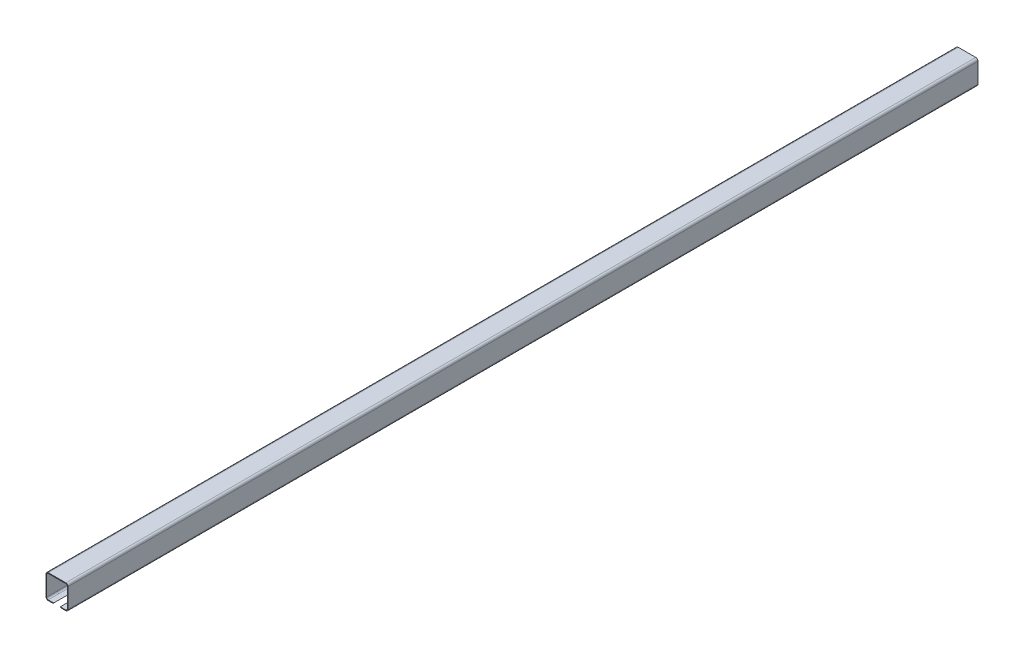
from build123d import *

# Parameters (mm, degrees)
BOSS_EXTRUDE1_DEPTH = 4135


with BuildPart() as part:
    # Sketch1 → Boss-Extrude1 (new body)
    with BuildSketch(Plane.XY):
        with BuildLine():
            Line((-40, 55), (0, 55))
            Line((0, 55), (40, 55))
            ThreePointArc((40, 55), (47.071067812, 52.071067812), (50, 45))
            Line((50, 45), (50, -45))
            ThreePointArc((50, -45), (47.071067812, -52.071067812), (40, -55))
            Line((40, -55), (18, -55))
            Line((18, -55), (15, -52))
            Line((15, -52), (40, -52))
            ThreePointArc((40, -52), (44.949747468, -49.949747468), (47, -45))
            Line((47, -45), (47, 45))
            ThreePointArc((47, 45), (44.949747468, 49.949747468), (40, 52))
            Line((40, 52), (0, 52))
            Line((0, 52), (-40, 52))
            ThreePointArc((-40, 52), (-44.949747468, 49.949747468), (-47, 45))
            Line((-47, 45), (-47, -45))
            ThreePointArc((-47, -45), (-44.949747468, -49.949747468), (-40, -52))
            Line((-40, -52), (-15, -52))
            Line((-15, -52), (-18, -55))
            Line((-18, -55), (-40, -55))
            ThreePointArc((-40, -55), (-47.071067812, -52.071067812), (-50, -45))
            Line((-50, -45), (-50, 45))
            ThreePointArc((-50, 45), (-47.071067812, 52.071067812), (-40, 55))
        make_face()
    extrude(amount=BOSS_EXTRUDE1_DEPTH)


solid = part.part
